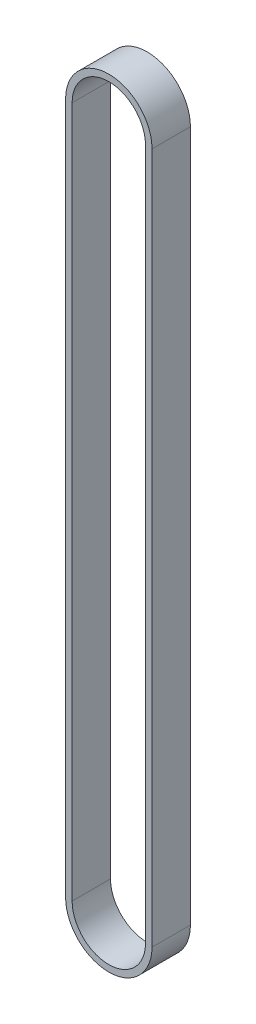
SolidWorks part; units mm, degrees
material "氯丁橡胶"
ref_plane "Front Plane" through (0, 0, 0) normal (0, 0, 1) x (1, 0, 0)
ref_plane "Top Plane" through (0, 0, 0) normal (0, 1, 0) x (1, 0, 0)
ref_plane "Right Plane" through (0, 0, 0) normal (1, 0, 0) x (0, 0, -1)
sketch "Sketch1" plane through (0, 0, 0) normal (0, 0, 1) x (1, 0, 0)
  line L0 (0, -54) -> (0, 54) construction
  line L1 (-6.75, -54) -> (-6.75, 54)
  line L2 (6.75, -54) -> (6.75, 54)
  line L3 (0, -54) -> (0, 54) construction
  line L4 (-5.73, -54) -> (-5.73, 54)
  line L5 (5.73, -54) -> (5.73, 54)
  arc A0 (-6.75, -54) -> (6.75, -54) centre (0, -54) ccw
  arc A1 (6.75, 54) -> (-6.75, 54) centre (0, 54) ccw
  arc A2 (-5.73, -54) -> (5.73, -54) centre (0, -54) ccw
  arc A3 (5.73, 54) -> (-5.73, 54) centre (0, 54) ccw
  point P2 (0, 0)
  point P9 (0, 0)
  dimension "D1" = 5.73
  dimension "D2" = 13.5
  dimension "D3" = 108
extrude "Boss-Extrude1" add sketch "Sketch1" along normal blind 6
